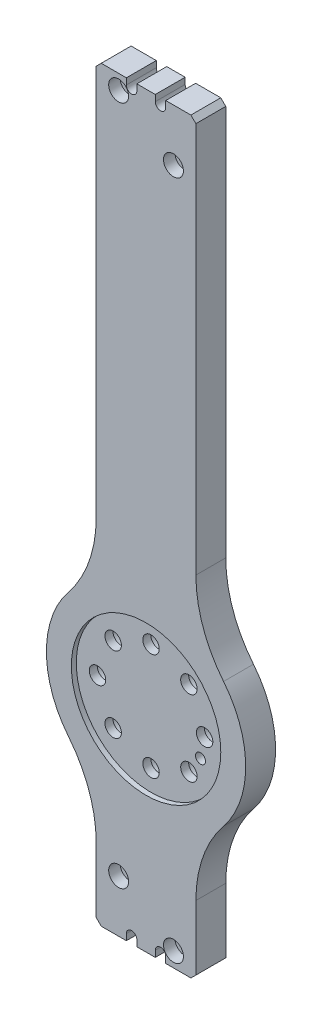
from build123d import *

# Parameters (mm, degrees)
SKETCH_1_W                   = 80
SKETCH_1_H                   = 300
EXTRUDE_1_DEPTH              = 12
CHAMFER_1_SIZE               = 2
SKETCH_2_R                   = 30
CUT_EXTRUDE_1_DEPTH          = 2
CUT_EXTRUDE_2_DEPTH          = 156.704848993
FILLET_1_R                   = 50
CHAMFER_3_SIZE               = 2
HOLE_WIZARD_M6_1_D           = 6.6
HOLE_WIZARD_M6_1_CBORE_D     = 11
HOLE_WIZARD_M6_1_CBORE_DEPTH = 6.8
F_4_0MM_1_D                  = 4
HOLE_WIZARD_M4_1_D           = 4.5
HOLE_WIZARD_M4_1_CBORE_D     = 8
HOLE_WIZARD_M4_1_CBORE_DEPTH = 4.6
CUT_EXTRUDE_3_DEPTH          = 156.704848993
PATTERN_CIRCULAR_1_COUNT     = 8


with BuildPart() as part:
    # 草图1 → 凸台-拉伸1 (new body)
    with BuildSketch(Plane.XY):
        Rectangle(SKETCH_1_W, SKETCH_1_H)
    extrude(amount=EXTRUDE_1_DEPTH)

    # 倒角1
    chamfer_1_edges = [part.edges().sort_by_distance(p)[0] for p in [
        (-40, -150, 6),
        (40, -150, 6),
        (40, 150, 6),
        (-40, 150, 6),
    ]]
    chamfer(chamfer_1_edges, length=CHAMFER_1_SIZE)

    # 草图2 → 切除-拉伸1 (cut)
    with BuildSketch(Plane.XY.offset(12)):
        with Locations((0, -65.5)):
            Circle(SKETCH_2_R)
    extrude(amount=-CUT_EXTRUDE_1_DEPTH, mode=Mode.SUBTRACT)

    # 草图3 → 切除-拉伸2 (cut, through all)
    with BuildSketch(Plane.XY.offset(12)):
        with BuildLine():
            Line((-38, -150), (-20, -150))
            Line((-20, -150), (-20, -100.141016151))
            ThreePointArc((-20, -100.141016151), (-34.641016151, -85.5), (-40, -65.5))
            Line((-40, -65.5), (-40, -148))
            Line((-40, -148), (-38, -150))
        make_face()
        with BuildLine():
            Line((20, -100.141016151), (20, -150))
            Line((20, -150), (38, -150))
            Line((38, -150), (40, -148))
            Line((40, -148), (40, -65.5))
            ThreePointArc((40, -65.5), (34.641016151, -85.5), (20, -100.141016151))
        make_face()
        with BuildLine():
            Line((-40, 148), (-40, -65.5))
            ThreePointArc((-40, -65.5), (-34.641016151, -45.5), (-20, -30.858983849))
            Line((-20, -30.858983849), (-20, 150))
            Line((-20, 150), (-38, 150))
            Line((-38, 150), (-40, 148))
        make_face()
        with BuildLine():
            ThreePointArc((20, -30.858983849), (34.641016151, -45.5), (40, -65.5))
            Line((40, -65.5), (40, 148))
            Line((40, 148), (38, 150))
            Line((38, 150), (20, 150))
            Line((20, 150), (20, -30.858983849))
        make_face()
    extrude(amount=-CUT_EXTRUDE_2_DEPTH, mode=Mode.SUBTRACT)

    # 圆角1
    fillet_1_edges = [part.edges().sort_by_distance(p)[0] for p in [
        (20, -30.858983849, 6),
        (-20, -30.858983849, 6),
        (-20, -100.141016151, 6),
        (20, -100.141016151, 6),
    ]]
    fillet(fillet_1_edges, radius=FILLET_1_R)

    # 倒角3
    chamfer_3_edges = [part.edges().sort_by_distance(p)[0] for p in [
        (20, -150, 6),
        (20, 150, 6),
        (-20, 150, 6),
        (-20, -150, 6),
    ]]
    chamfer(chamfer_3_edges, length=CHAMFER_3_SIZE)

    # M6 六角圆柱头螺钉的柱形沉头孔1 (through all)
    with Locations(Plane(origin=(0, 0, 0), x_dir=(-1, 0, 0), z_dir=(0, 0, -1))):
        with Locations((0, -87)):
            hole_wizard_m6_1 = CounterBoreHole(HOLE_WIZARD_M6_1_D / 2, HOLE_WIZARD_M6_1_CBORE_D / 2, HOLE_WIZARD_M6_1_CBORE_DEPTH)

    # Ø4.0mm 暗销孔1 (through all)
    with Locations(Plane(origin=(0, 0, 0), x_dir=(-1, 0, 0), z_dir=(0, 0, -1))):
        with Locations((-19.863409949, -73.727693796)):
            Hole(F_4_0MM_1_D / 2)

    # M4 六角圆柱头螺钉的柱形沉头孔1 (through all)
    with Locations(Plane.XY.offset(12)):
        with Locations((-11, -129.05), (11, -144.05), (-11, 144.05), (11, 129.05)):
            CounterBoreHole(HOLE_WIZARD_M4_1_D / 2, HOLE_WIZARD_M4_1_CBORE_D / 2, HOLE_WIZARD_M4_1_CBORE_DEPTH)

    # 草图14 → 切除-拉伸3 (cut, through all)
    with BuildSketch(Plane.XY.offset(12)):
        with BuildLine():
            Line((7.9, -147.5), (7.9, -150))
            ThreePointArc((7.9, -150), (5.8, -152.1), (3.7, -150))
            Line((3.7, -150), (3.7, -147.5))
            ThreePointArc((3.7, -147.5), (5.8, -145.4), (7.9, -147.5))
        make_face()
        with BuildLine():
            Line((-3.7, -147.5), (-3.7, -150))
            ThreePointArc((-3.7, -150), (-5.8, -152.1), (-7.9, -150))
            Line((-7.9, -150), (-7.9, -147.5))
            ThreePointArc((-7.9, -147.5), (-5.8, -145.4), (-3.7, -147.5))
        make_face()
        with BuildLine():
            Line((7.9, 147.5), (7.9, 150))
            ThreePointArc((7.9, 150), (5.8, 152.1), (3.7, 150))
            Line((3.7, 150), (3.7, 147.5))
            ThreePointArc((3.7, 147.5), (5.8, 145.4), (7.9, 147.5))
        make_face()
        with BuildLine():
            Line((-3.7, 147.5), (-3.7, 150))
            ThreePointArc((-3.7, 150), (-5.8, 152.1), (-7.9, 150))
            Line((-7.9, 150), (-7.9, 147.5))
            ThreePointArc((-7.9, 147.5), (-5.8, 145.4), (-3.7, 147.5))
        make_face()
    extrude(amount=-CUT_EXTRUDE_3_DEPTH, mode=Mode.SUBTRACT)

    # 阵列(圆周)1: M6 六角圆柱头螺钉的柱形沉头孔1 ×8 about axis
    pattern_circular_1_axis = Axis((0, -65.5, 0), (0, 0, 1))
    for i in range(1, PATTERN_CIRCULAR_1_COUNT):
        add(hole_wizard_m6_1.rotate(pattern_circular_1_axis, i * 360 / PATTERN_CIRCULAR_1_COUNT), mode=Mode.SUBTRACT)


solid = part.part
